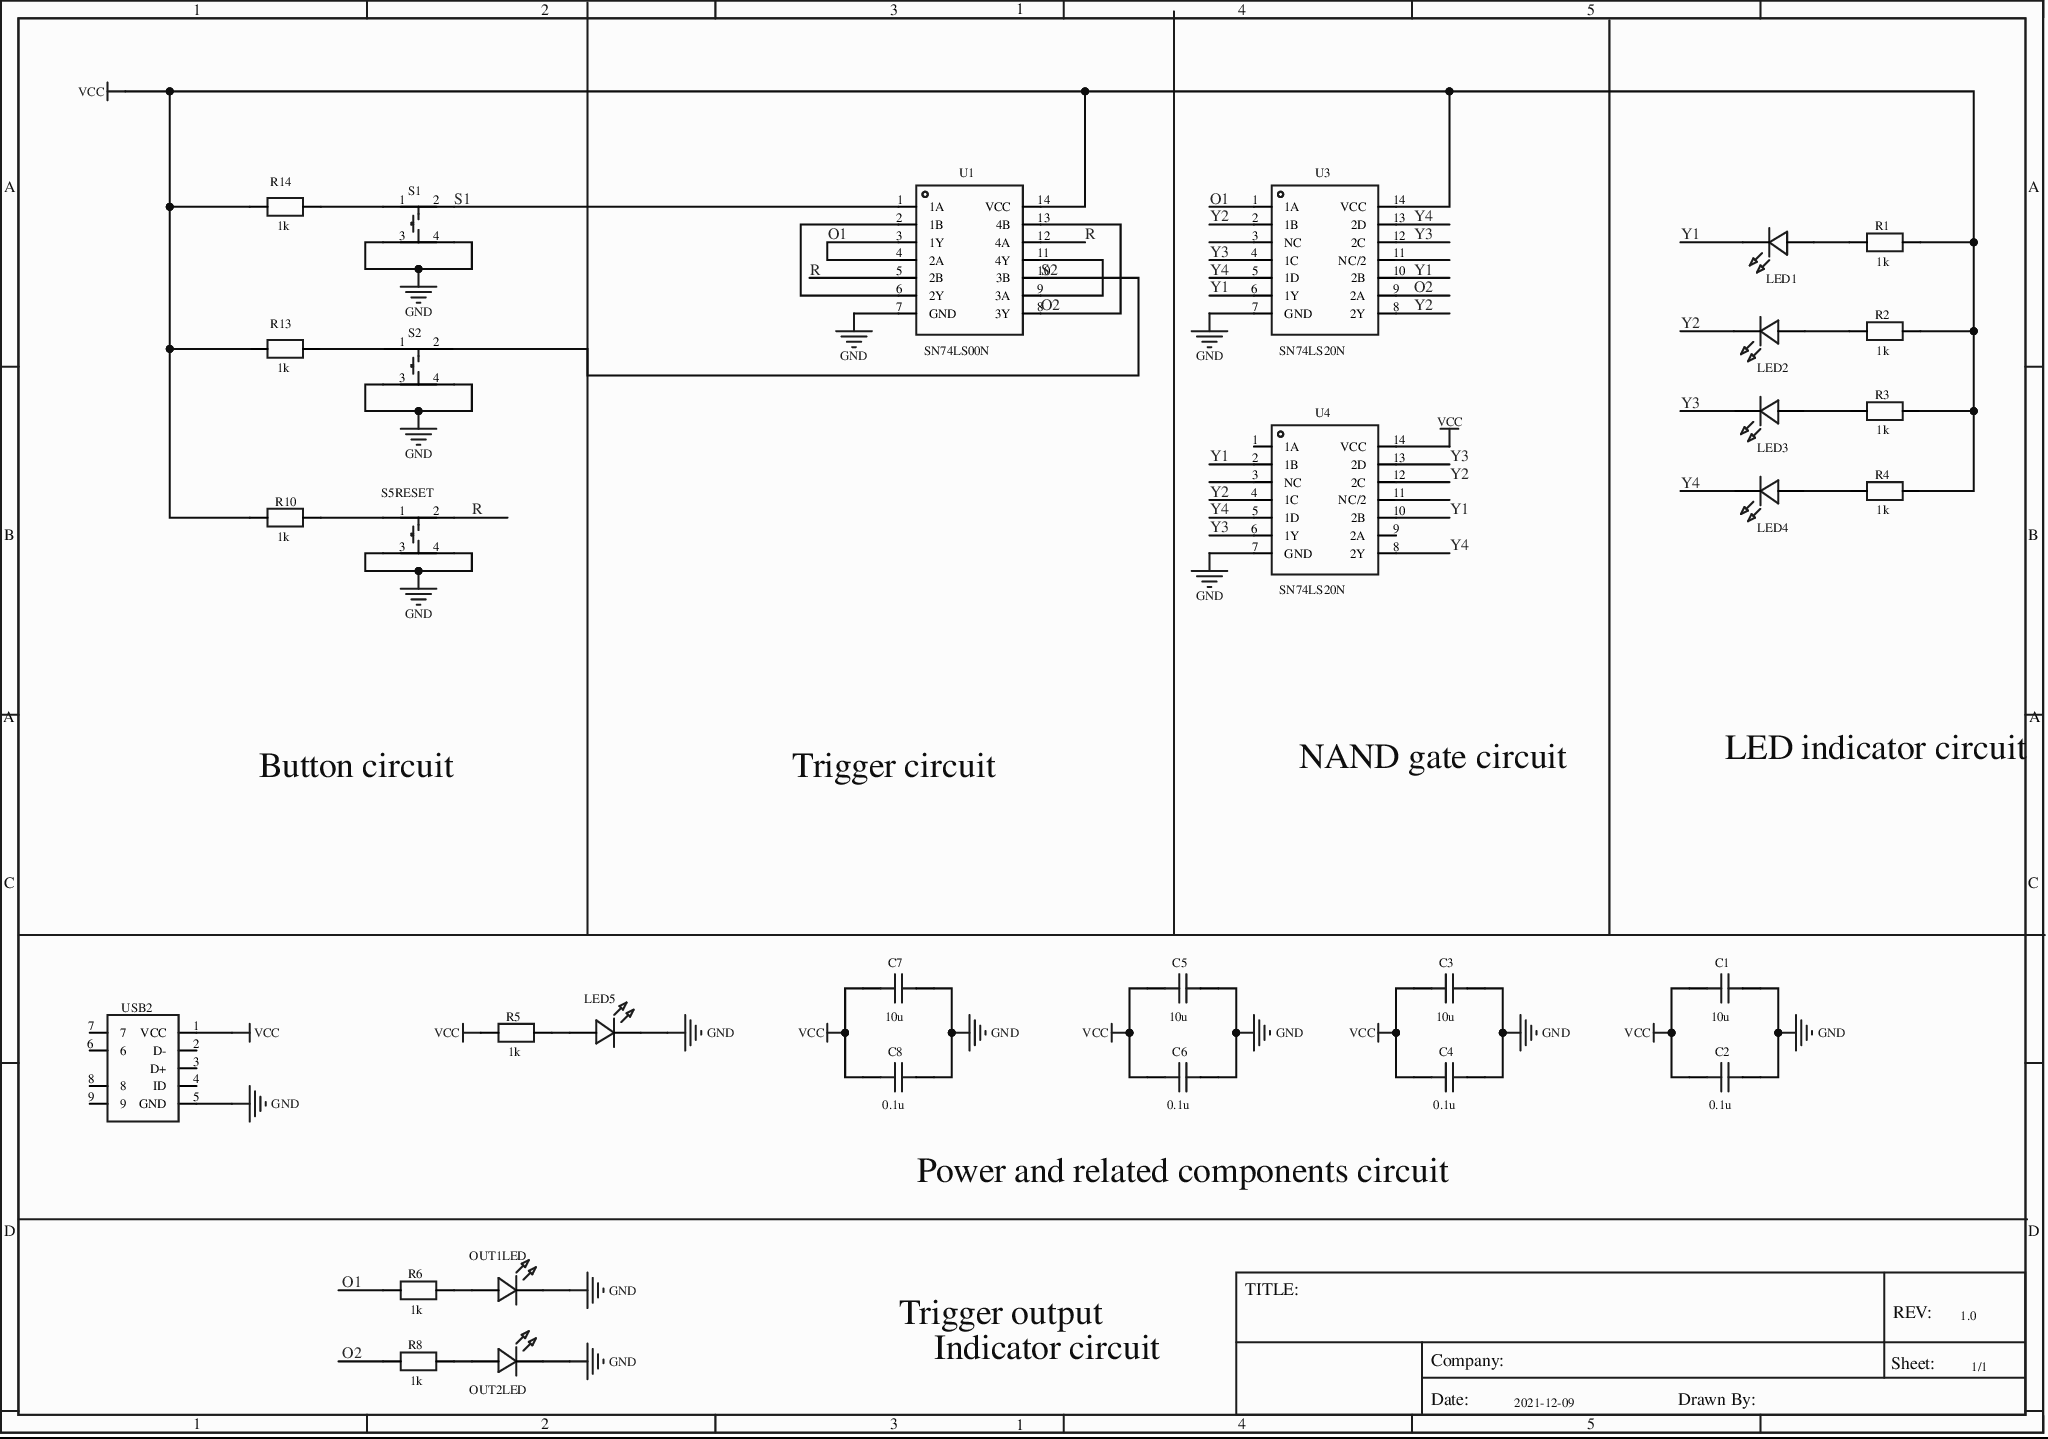
[diagram p0: MISC75096-3.schdoc]
# Altium project MISC75096-2.PrjPcb
1 sheet, 32 parts. Net scope: global (net labels, ports and power ports of the same name join across sheets).
Board file: MISC75096.pcbdoc

## Sheet MISC75096-3.schdoc
size 292 x 204 mm; Name: MISC75096; @Project Name: MISC75096; REV: 1.0; Date: 2021-12-09; Sheet: 1/1; @Page No: 1; @Page Count: 1; @Schematic Name: MISC75096; @Board Name: MISC75096; @Update Date: 2025-05-06; @Create Time: 21:51:02; @Update Time: 21:51:06; @Create Date: 2025-05-06

### Parts
C1  10u  [C0805]
C2  0.1u  [C0805]
C3  10u  [C0805]
C4  0.1u  [C0805]
C5  10u  [C0805]
C6  0.1u  [C0805]
C7  10u  [C0805]
C8  0.1u  [C0805]
LED1  LED-TH-5mm_R  [LED-TH_BD5.0_RED]  (value not drawn)
LED2  LED-TH-5mm_R  [LED-TH_BD5.0_RED]  (value not drawn)
LED3  LED-TH-5mm_R  [LED-TH_BD5.0_RED]  (value not drawn)
LED4  LED-TH-5mm_R  [LED-TH_BD5.0_RED]  (value not drawn)
LED5  LED-TH-3mm_R  [LED-TH_BD3.0_RED]  (value not drawn)
OUT1LED  LED-TH-5mm_R  [LED-TH_BD5.0_RED]  (value not drawn)
OUT2LED  LED-TH-5mm_R  [LED-TH_BD5.0_RED]  (value not drawn)
R1  1k  [R0805]
R2  1k  [R0805]
R3  1k  [R0805]
R4  1k  [R0805]
R5  1k  [R0805]
R6  1k  [R0805]
R8  1k  [R0805]
R10  1k  [R0805]
R13  1k  [R0805]
R14  1k  [R0805]
S1  TC-1157-B-A  [KEY-TH_4P-L6.4-W6.0-P4.50-LS7.3-TL]  (value not drawn)
S2  TC-1157-B-A  [KEY-TH_4P-L6.4-W6.0-P4.50-LS7.3-TL]  (value not drawn)
S5RESET  TC-1157-B-A  [KEY-TH_4P-L6.4-W6.0-P4.50-LS7.3-TL]  (value not drawn)
U1  SN74LS00N  [PDIP-14_L19.7-W6.6-P2.54-LS8.3-BL]
U3  SN74LS20N  [DIP-14_L19.0-W7.0-P2.54-LS7.6-BL]
U4  SN74LS20N  [DIP-14_L19.0-W7.0-P2.54-LS7.6-BL]
USB2  U-F-M5DD-W-2-SUS  [MICRO-USB-SMD_U-F-M5DD-W-2-SUS]  (value not drawn)

### Nets
GND: C1.2 C2.2 C3.2 C4.2 C5.2 C6.2 C7.2 C8.2 LED5.2 OUT1LED.2 OUT2LED.2 S1.3 S1.4 S2.3 S2.4 S5RESET.3 S5RESET.4 U1.7(GND) U3.7(GND) U4.7(GND) USB2.5(GND)
VCC: C1.1 C2.1 C3.1 C4.1 C5.1 C6.1 C7.1 C8.1 R1.2 R2.2 R3.2 R4.2 R5.1 R10.1 R13.1 R14.1 U1.14(VCC) U3.14(VCC) U4.14(VCC) USB2.1(VCC)
O1: R6.1 U1.3(1Y) U1.4(2A) U3.1(1A)
O2: R8.1 U1.8(3Y) U1.13(4B) U3.9(2A)
R: S5RESET.2 U1.5(2B) U1.12(4A)
S1: S1.2 U1.1(1A)
S2: S2.2 U1.10(3B)
Y1: LED1.2 U3.6(1Y) U3.10(2B) U4.2(1B) U4.10(2B)
Y2: LED2.2 U3.2(1B) U3.8(2Y) U4.4(1C) U4.12(2C)
Y3: LED3.2 U3.4(1C) U3.12(2C) U4.6(1Y) U4.13(2D)
Y4: LED4.2 U3.5(1D) U3.13(2D) U4.5(1D) U4.8(2Y)
NetLED1_1: LED1.1 R1.1
NetLED2_1: LED2.1 R2.1
NetLED3_1: LED3.1 R3.1
NetLED4_1: LED4.1 R4.1
NetLED5_1: LED5.1 R5.2
NetOUT1LED_1: OUT1LED.1 R6.2
NetOUT2LED_1: OUT2LED.1 R8.2
NetR10_2: R10.2 S5RESET.1
NetR13_2: R13.2 S2.1
NetR14_2: R14.2 S1.1
NetU1_2: U1.2(1B) U1.6(2Y)
NetU1_9: U1.9(3A) U1.11(4Y)

Not connected (* = marked no-connect by the designer): U3 3(NC) 11(NC/2); U4 1(1A) 3(NC) 9(2A) 11(NC/2); USB2 2(D-)* 3(D+)* 4(ID)* 6* 7* 8* 9*

### Notes on the sheet
- LED indicator circuit
- Button circuit
- Trigger circuit
- NAND gate circuit
- Power and related components circuit
- Trigger output
- Indicator circuit
- 1
- 2
- 3
- 4
- 5
- A
- B
- C
- D
- TITLE:
- Company:
- Sheet:
- REV:
- 1.0
- 1/1
- Date:
- 2021-12-09
- Drawn By:

### Library data of the parts
C1 C3 C5 C7 = 10u: Convert to PCB: yes; Origin Footprint: C0805; Device: 10u; Symbol: 10u; Add into BOM: yes; Supplier: LCSC; FootprintName: C0805
C2 C4 C6 C8 = 0.1u: Convert to PCB: yes; Origin Footprint: C0805; Device: 0.1u; Symbol: 0.1u; Add into BOM: yes; FootprintName: C0805
LED1-LED4 OUT1LED OUT2LED = 333-2SURD/S530-A3: Manufacturer: EVERLIGHT(台湾亿光); Convert to PCB: yes; Origin Footprint: LED-TH_BD5.0_RED; Device: 333-2SURD/S530-A3; Symbol: LED-TH-5mm_R; Add into BOM: yes; ManufacturerPart: 333-2SURD/S530-A3; SupplierPart: C87271; Supplier: LCSC; FootprintName: LED-TH_BD5.0_RED
LED5 = 204-10SDRD/S530-A3-L: Manufacturer: EVERLIGHT(台湾亿光); Convert to PCB: yes; Origin Footprint: LED-TH_BD3.0_RED; Device: 204-10SDRD/S530-A3-L; Symbol: LED-TH-3mm_R; Add into BOM: yes; ManufacturerPart: 204-10SDRD/S530-A3-L; SupplierPart: C84774; Supplier: LCSC; FootprintName: LED-TH_BD3.0_RED
R1-R6 R8 R10 R13 R14 = 1k: Convert to PCB: yes; Origin Footprint: R0805; Device: 1k; Symbol: 1k; Add into BOM: yes; Supplier: LCSC; FootprintName: R0805
S1 S2 S5RESET = TC-1157-B-A: Manufacturer: XKB Enterprise; Convert to PCB: yes; Origin Footprint: KEY-TH_4P-L6.4-W6.0-P4.50-LS7.3-TL; Device: TC-1157-B-A; Symbol: TC-1157-B-A; Add into BOM: yes; Supplier: LCSC; SupplierPart: C500077; ManufacturerPart: TC-1157-B-A; JLCPCB Part Class: Extended Part; FootprintName: KEY-TH_4P-L6.4-W6.0-P4.50-LS7.3-TL
U1 = SN74LS00N: Manufacturer: TI; Convert to PCB: yes; Origin Footprint: PDIP-14_L19.7-W6.6-P2.54-LS8.3-BL; Device: SN74LS00N; Symbol: SN74LS00N; Add into BOM: yes; Supplier: LCSC; ManufacturerPart: SN74LS00N; SupplierPart: C181629; JLCPCB Part Class: Extended Part; FootprintName: PDIP-14_L19.7-W6.6-P2.54-LS8.3-BL
U3 U4 = SN74LS20N: Manufacturer: TI; Convert to PCB: yes; Origin Footprint: DIP-14_L19.0-W7.0-P2.54-LS7.6-BL; Device: SN74LS20N; Symbol: SN74LS20N; Add into BOM: yes; Supplier: LCSC; ManufacturerPart: SN74LS20N; SupplierPart: C133588; JLCPCB Part Class: Extended Part; FootprintName: DIP-14_L19.0-W7.0-P2.54-LS7.6-BL
USB2 = U-F-M5DD-W-2-SUS: Manufacturer: Korean Hroparts Elec; Convert to PCB: yes; Origin Footprint: MICRO-USB-SMD_U-F-M5DD-W-2-SUS; Device: U-F-M5DD-W-2-SUS; Symbol: U-F-M5DD-W-2-SUS; Add into BOM: yes; Supplier: LCSC; SupplierPart: C879723; ManufacturerPart: U-F-M5DD-W-2-SUS; JLCPCB Part Class: Extended Part; FootprintName: MICRO-USB-SMD_U-F-M5DD-W-2-SUS